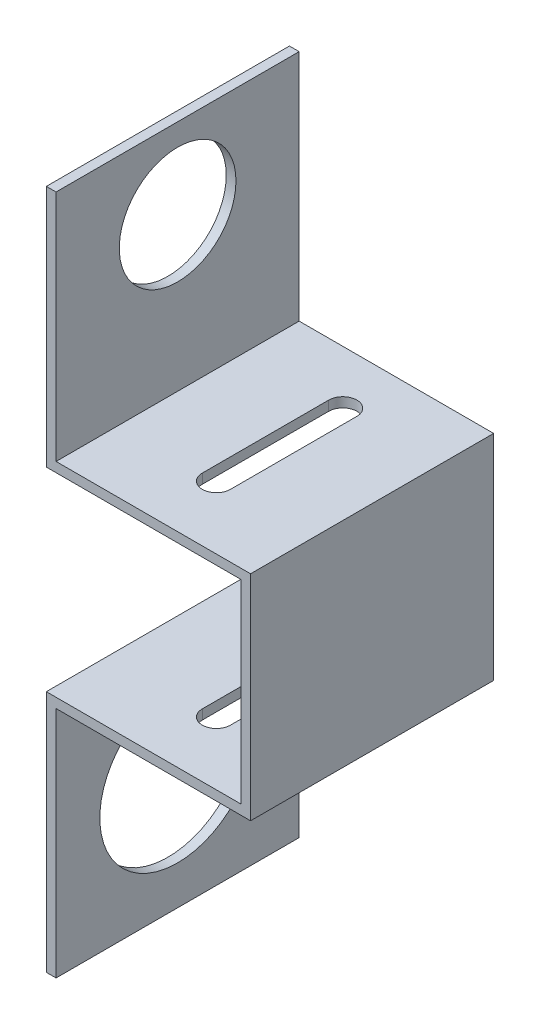
SolidWorks part; units mm, degrees
ref_plane "Front Plane" through (0, 0, 0) normal (0, 0, 1) x (1, 0, 0)
ref_plane "Top Plane" through (0, 0, 0) normal (0, 1, 0) x (1, 0, 0)
ref_plane "Right Plane" through (0, 0, 0) normal (1, 0, 0) x (0, 0, -1)
sketch "Sketch1" plane through (0, 0, 0) normal (0, 0, 1) x (1, 0, 0)
  line L0 (0, 50) -> (0, 0)
  line L1 (0, 0) -> (40, 0)
  line L2 (40, 0) -> (40, -40)
  line L3 (40, -40) -> (0, -40)
  line L4 (0, -40) -> (0, -90)
  line L5 (2, 50) -> (2, 2)
  line L6 (2, 2) -> (42, 2)
  line L7 (42, 2) -> (42, -42)
  line L8 (42, -42) -> (2, -42)
  line L9 (2, -42) -> (2, -90)
  line L10 (0, 50) -> (2, 50)
  line L11 (0, -90) -> (2, -90)
  dimension "D1" = 2
extrude "Boss-Extrude1" add sketch "Sketch1" along normal blind 50
sketch "Sketch2" plane through (0, 2, 0) normal (0, 1, 0) x (1, 0, 0)
  line L0 (22, 0) -> (22, -50) construction
  line L1 (42, 0) -> (2, 0) construction
  line L2 (42, -50) -> (2, -50) construction
  line L3 (22, -11.0266) -> (22, -37.0294) construction
  line L4 (24.8983, -11.0266) -> (24.8983, -37.0294)
  line L5 (19.1017, -11.0266) -> (19.1017, -37.0294)
  arc A0 (24.8983, -11.0266) -> (19.1017, -11.0266) centre (22, -11.0266) ccw
  arc A1 (19.1017, -37.0294) -> (24.8983, -37.0294) centre (22, -37.0294) ccw
  point P8 (22, -24.028)
extrude "Cut-Extrude1" cut sketch "Sketch2" against normal blind 50
sketch "Sketch3" plane through (2, 0, 0) normal (1, 0, 0) x (0, 0, -1)
  circle A0 centre (-25, -66) radius 16
extrude "Cut-Extrude2" cut sketch "Sketch3" against normal blind 50
sketch "Sketch4" plane through (2, 0, 0) normal (1, 0, 0) x (0, 0, -1)
  circle A0 centre (-25, 33.4735) radius 12
extrude "Cut-Extrude3" cut sketch "Sketch4" against normal blind 50
